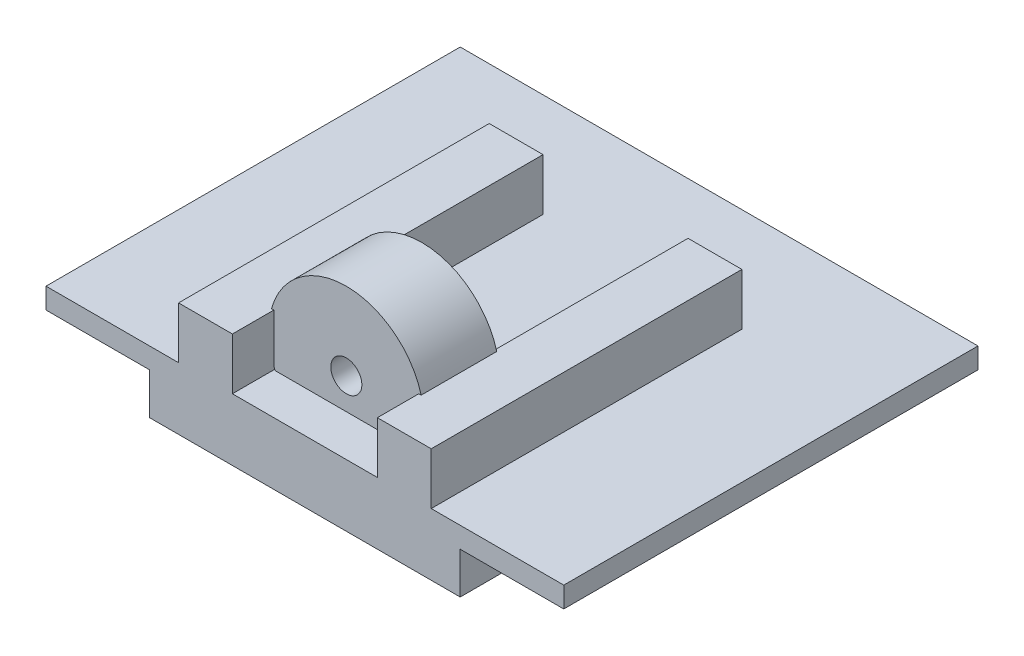
SolidWorks part; units mm, degrees
ref_plane "Front Plane" through (0, 0, 0) normal (0, 0, 1) x (1, 0, 0)
ref_plane "Top Plane" through (0, 0, 0) normal (0, 1, 0) x (1, 0, 0)
ref_plane "Right Plane" through (0, 0, 0) normal (1, 0, 0) x (0, 0, -1)
sketch "Sketch1" plane through (0, 0, 0) normal (0, 1, 0) x (1, 0, 0)
  line L1 (-250, 200) -> (250, 200)
  line L2 (-250, 200) -> (-250, -200)
  line L3 (-250, -200) -> (250, -200)
  line L4 (250, 200) -> (250, -200)
  line L5 (-250, 200) -> (250, -200) construction
  line L6 (-250, -200) -> (250, 200) construction
  point P0 (0, 0)
  dimension "D1" = 500
  dimension "D2" = 400
extrude "Boss-Extrude1" add sketch "Sketch1" along normal blind 20
sketch "Sketch2" plane through (0, 20, 0) normal (0, 1, 0) x (1, 0, 0)
  line L0 (0, 200) -> (0, -118.8316) construction
  line L1 (250, 200) -> (-250, 200) construction
  line L2 (-70, 100) -> (-70, -200)
  line L3 (122, 100) -> (70, 100)
  line L4 (122, 100) -> (122, -200)
  line L5 (122, -200) -> (70, -200)
  line L6 (70, 100) -> (70, -200)
  line L7 (-122, -200) -> (-70, -200)
  line L8 (-122, 100) -> (-122, -200)
  line L9 (-122, 100) -> (-70, 100)
  line L10 (-250, -200) -> (250, -200) construction
  dimension "D1" = 300
  dimension "D2" = 52
  dimension "D3" = 140
extrude "Boss-Extrude2" add sketch "Sketch2" along normal blind 50
sketch "Sketch3" plane through (0, 0, 0) normal (0, -1, 0) x (1, 0, 0)
  line L0 (-250, 200) -> (250, 200) construction
  line L1 (-150, -200) -> (150, -200)
  line L2 (-150, -200) -> (-150, 200)
  line L3 (-150, 200) -> (150, 200)
  line L4 (150, -200) -> (150, 200)
  line L5 (-150, -200) -> (150, 200) construction
  line L6 (-150, 200) -> (150, -200) construction
  point P0 (0, 0)
  dimension "D1" = 300
extrude "Boss-Extrude3" add sketch "Sketch3" along normal blind 40
ref_plane "Plane1" through (0, 0, 160) normal (0, 0, 1) x (1, 0, 0)
sketch "Sketch6" plane through (0, 0, 160) normal (0, 0, 1) x (1, 0, 0)
  line L0 (150, -40) -> (-150, -40) construction
  circle A0 centre (0, 50) radius 75
  dimension "D1" = 150
  dimension "D2" = 90
extrude "Boss-Extrude5" add sketch "Sketch6" against normal blind 73
sketch "Sketch7" plane through (0, 0, 160) normal (0, 0, 1) x (1, 0, 0)
  circle A0 centre (0, 50) radius 15
  dimension "D1" = 30
extrude "Cut-Extrude2" cut sketch "Sketch7" against normal through all
